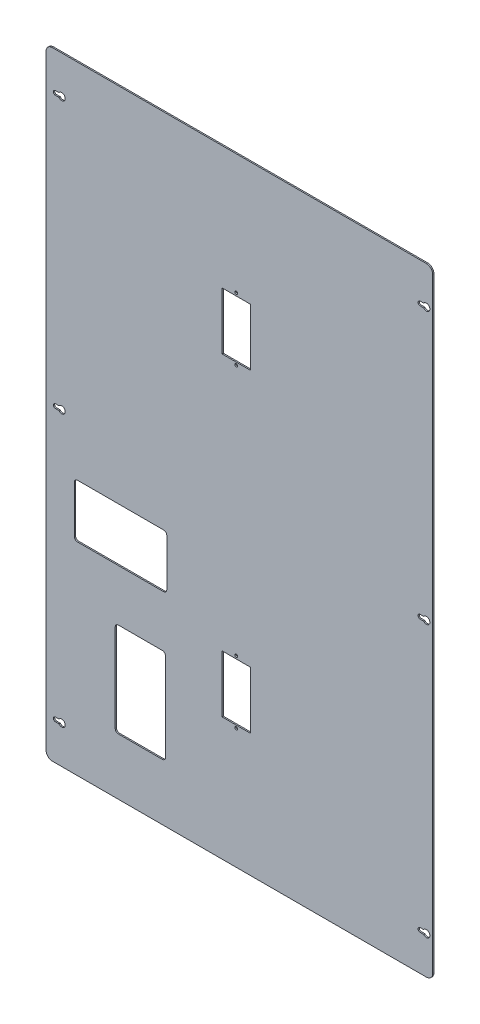
from build123d import *

# Parameters (mm, degrees)
SKETCH1_W            = 615
SKETCH1_H            = 983
BOSS_EXTRUDE1_DEPTH  = 2
SKETCH7_W            = 45
SKETCH7_H            = 91
CUT_EXTRUDE4_DEPTH   = 580.76935069
SKETCH8_R            = 2.25
CUT_EXTRUDE5_DEPTH   = 580.76935069
FILLET3_R            = 10
CUT_EXTRUDE6_DEPTH   = 10
LPATTERN1_COUNT      = 3
LPATTERN1_PITCH      = 431.5
LPATTERN1_COUNT_DIR2 = 2
LPATTERN1_PITCH_DIR2 = 580
SKETCH12_W           = 80
SKETCH12_H           = 150
CUT_EXTRUDE8_DEPTH   = 580.76935069
SKETCH13_W           = 147
SKETCH13_H           = 85
CUT_EXTRUDE9_DEPTH   = 10
FILLET4_R            = 5


with BuildPart() as part:
    # Sketch1 → Boss-Extrude1 (new body)
    with BuildSketch(Plane.XY):
        Rectangle(SKETCH1_W, SKETCH1_H)
    extrude(amount=BOSS_EXTRUDE1_DEPTH)

    # Sketch7 → Cut-Extrude4 (cut, through all)
    with BuildSketch(Plane(origin=(0, 0, 0), x_dir=(-1, 0, 0), z_dir=(0, 0, -1))):
        with Locations((5, 250)):
            Rectangle(SKETCH7_W, SKETCH7_H)
        with Locations((5, -250)):
            Rectangle(SKETCH7_W, SKETCH7_H)
    extrude(amount=-CUT_EXTRUDE4_DEPTH, mode=Mode.SUBTRACT)

    # Sketch8 → Cut-Extrude5 (cut, through all)
    with BuildSketch(Plane(origin=(0, 0, 0), x_dir=(-1, 0, 0), z_dir=(0, 0, -1))):
        with Locations((5, 300)):
            Circle(SKETCH8_R)
        with Locations((5, 200)):
            Circle(SKETCH8_R)
        with Locations((5, -200)):
            Circle(SKETCH8_R)
        with Locations((5, -300)):
            Circle(SKETCH8_R)
    extrude(amount=-CUT_EXTRUDE5_DEPTH, mode=Mode.SUBTRACT)

    # Fillet3
    fillet3_edges = [part.edges().sort_by_distance(p)[0] for p in [
        (307.5, -491.5, 1),
        (-307.5, -491.5, 1),
        (-307.5, 491.5, 1),
        (307.5, 491.5, 1),
    ]]
    fillet(fillet3_edges, radius=FILLET3_R)

    # Sketch10 → Cut-Extrude6 (cut)
    with BuildSketch(Plane(origin=(0, 0, 0), x_dir=(-1, 0, 0), z_dir=(0, 0, -1))):
        with BuildLine():
            Line((292.5, 434.8), (286.9, 434.8))
            ThreePointArc((286.9, 434.8), (277, 431.5), (286.9, 428.2))
            Line((286.9, 428.2), (292.5, 428.2))
            ThreePointArc((292.5, 428.2), (295.8, 431.5), (292.5, 434.8))
        make_face()
    cut_extrude6 = extrude(amount=-CUT_EXTRUDE6_DEPTH, mode=Mode.SUBTRACT)

    # LPattern1: Cut-Extrude6 3 × 2
    with Locations(*[(j * LPATTERN1_PITCH_DIR2, -i * LPATTERN1_PITCH, 0) for i in range(LPATTERN1_COUNT) for j in range(LPATTERN1_COUNT_DIR2) if (i, j) != (0, 0)]):
        add(cut_extrude6, mode=Mode.SUBTRACT)

    # Sketch12 → Cut-Extrude8 (cut, through all)
    with BuildSketch(Plane.XY.offset(2)):
        with Locations((-157.5, -326.5)):
            Rectangle(SKETCH12_W, SKETCH12_H)
    extrude(amount=-CUT_EXTRUDE8_DEPTH, mode=Mode.SUBTRACT)

    # Sketch13 → Cut-Extrude9 (cut)
    with BuildSketch(Plane(origin=(0, 0, 0), x_dir=(-1, 0, 0), z_dir=(0, 0, -1))):
        with Locations((189, -127)):
            Rectangle(SKETCH13_W, SKETCH13_H)
    extrude(amount=-CUT_EXTRUDE9_DEPTH, mode=Mode.SUBTRACT)

    # Fillet4
    fillet4_edges = [part.edges().sort_by_distance(p)[0] for p in [
        (-197.5, -401.5, 1),
        (-197.5, -251.5, 1),
        (-117.5, -251.5, 1),
        (-117.5, -401.5, 1),
        (-115.5, -169.5, 1),
        (-115.5, -84.5, 1),
        (-262.5, -84.5, 1),
        (-262.5, -169.5, 1),
    ]]
    fillet(fillet4_edges, radius=FILLET4_R)


solid = part.part
